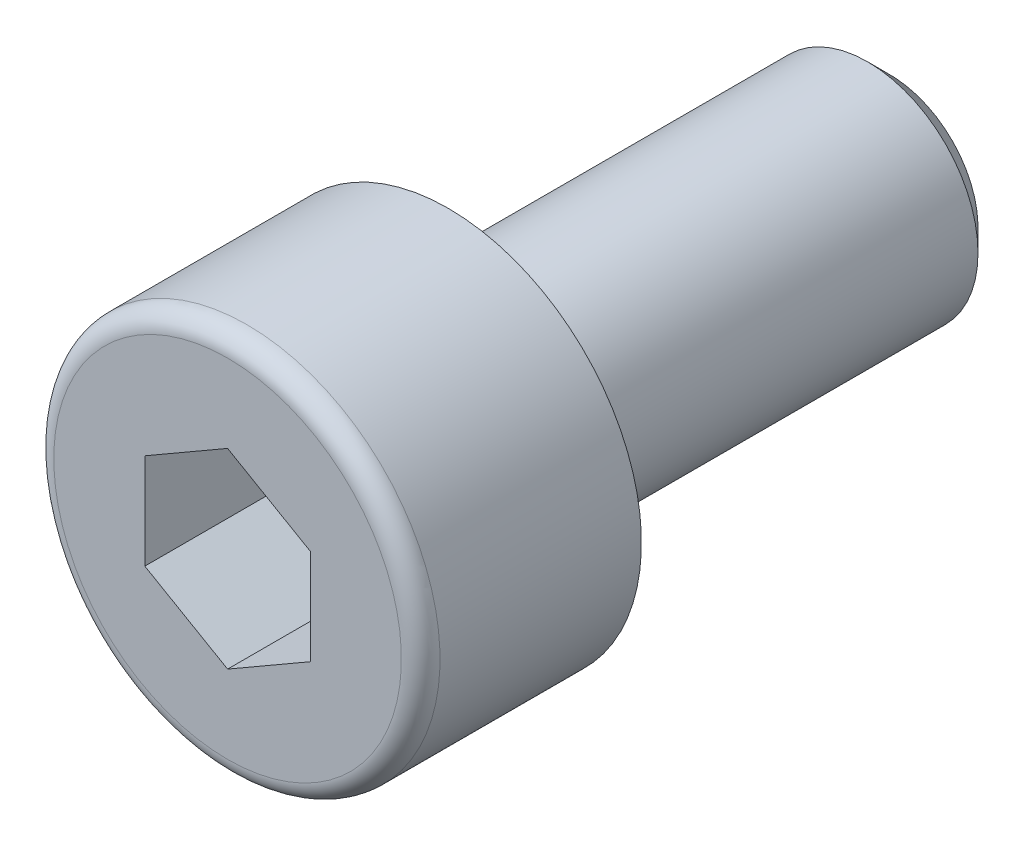
from build123d import *

# Parameters (mm, degrees)
CUT_EXTRUDE_1_DEPTH = 2.45
FILLET_1_R          = 0.35
CHAMFER_1_SIZE      = 0.4


with BuildPart() as part:
    # 草图3 → 旋转1 (revolve)
    with BuildSketch(Plane(origin=(0, 0, 0), x_dir=(0, 0, -1), z_dir=(1, 0, 0)), mode=Mode.PRIVATE) as revolve_1_sk:
        Polygon((-4, 0), (-4, 3.5), (0, 3.5), (0, 2), (8, 2), (8, 0), align=None)
    revolve(revolve_1_sk.sketch.rotate(Axis((0, 0, 4), (0, 0, -1)), 180), axis=Axis((0, 0, 4), (0, 0, -1)))

    # 草图4 → 切除-拉伸1 (cut)
    with BuildSketch(Plane.XY.offset(4)):
        Polygon((0, 1.732050808), (-1.5, 0.866025404), (-1.5, -0.866025404), (0, -1.732050808), (1.5, -0.866025404), (1.5, 0.866025404), align=None)
    extrude(amount=-CUT_EXTRUDE_1_DEPTH, mode=Mode.SUBTRACT)

    # 圆角1
    fillet_1_edges = [part.edges().sort_by_distance(p)[0] for p in [
        (0, 3.5, 4),
    ]]
    fillet(fillet_1_edges, radius=FILLET_1_R)

    # 倒角1
    chamfer_1_edges = [part.edges().sort_by_distance(p)[0] for p in [
        (0, 2, -8),
    ]]
    chamfer(chamfer_1_edges, length=CHAMFER_1_SIZE)


solid = part.part
